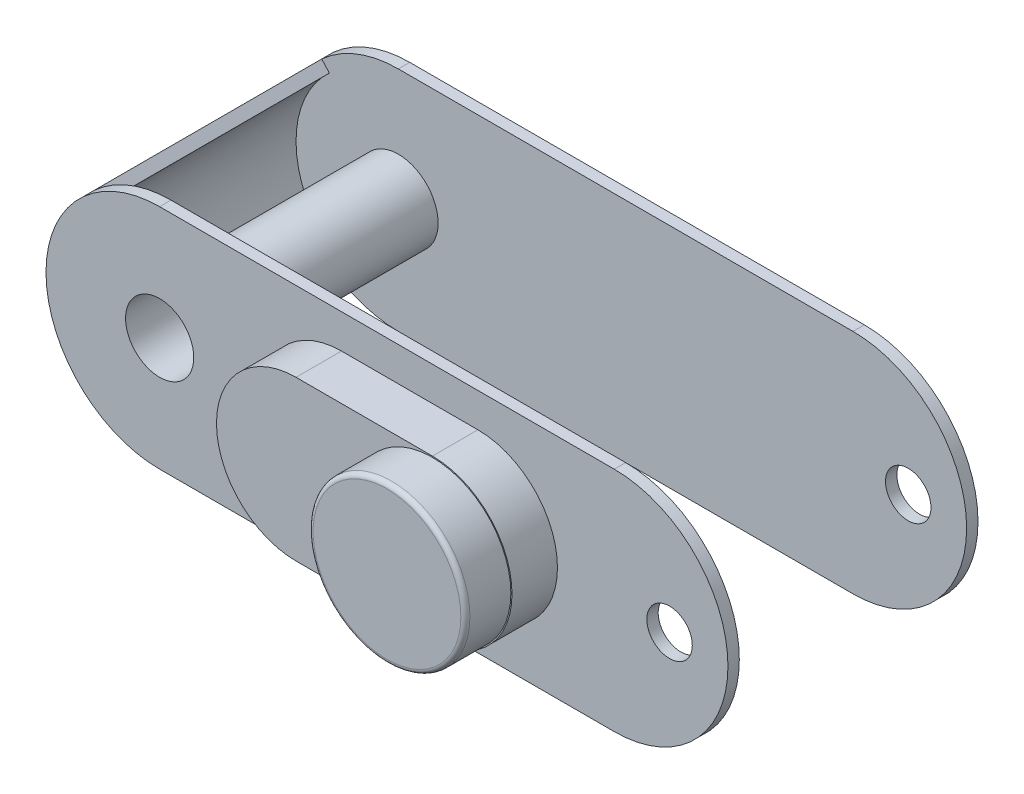
from build123d import *

# Parameters (mm, degrees)
SKETCH5_R           = 15
BOSS_EXTRUDE2_DEPTH = 5
BOSS_EXTRUDE3_START = 100
SKETCH6_R           = 15
BOSS_EXTRUDE3_DEPTH = 5
SKETCH7_R           = 17.5
SKETCH7_R_2         = 15
BOSS_EXTRUDE4_DEPTH = 100
SKETCH8_R           = 10
CUT_EXTRUDE1_DEPTH  = 46
BOSS_EXTRUDE5_DEPTH = 20
SKETCH10_R          = 34.5
BOSS_EXTRUDE6_DEPTH = 20
SKETCH11_R          = 10
CUT_EXTRUDE2_DEPTH  = 127
BOSS_EXTRUDE8_REACH = 295.3
FILLET1_R           = 2


with BuildPart() as part:
    # Sketch5 → Boss-Extrude2 (new body)
    with BuildSketch(Plane.XY):
        with BuildLine():
            Line((0, 50), (200, 50))
            ThreePointArc((200, 50), (250, 0), (200, -50))
            Line((200, -50), (0, -50))
            ThreePointArc((0, -50), (-50, 0), (0, 50))
        make_face()
        Circle(SKETCH5_R, mode=Mode.SUBTRACT)
    extrude(amount=BOSS_EXTRUDE2_DEPTH)



with BuildPart() as body_2:
    # Sketch6 → Boss-Extrude3 (new body)
    with BuildSketch(Plane.XY.offset(5).offset(BOSS_EXTRUDE3_START)):
        with BuildLine():
            Line((0, -50), (200, -50))
            ThreePointArc((200, -50), (250, 0), (200, 50))
            Line((200, 50), (0, 50))
            ThreePointArc((0, 50), (-50, 0), (0, -50))
        make_face()
        Circle(SKETCH6_R, mode=Mode.SUBTRACT)
    extrude(amount=BOSS_EXTRUDE3_DEPTH)


with BuildPart() as part_1:
    add(part.part)

    add(body_2.part)  # Boss-Extrude4 merges body 2
    # Sketch7 → Boss-Extrude4 (add)
    with BuildSketch(Plane.XY.offset(5)):
        Circle(SKETCH7_R)
        Circle(SKETCH7_R_2, mode=Mode.SUBTRACT)
    extrude(amount=BOSS_EXTRUDE4_DEPTH)

    # Sketch8 → Cut-Extrude1 (cut)
    with BuildSketch(Plane(origin=(0, 0, 105), x_dir=(-1, 0, 0), z_dir=(0, 0, -1))):
        with Locations((-80, 0)):
            Circle(SKETCH8_R)
        with Locations((-140, 0)):
            Circle(SKETCH8_R)
    extrude(amount=-CUT_EXTRUDE1_DEPTH, mode=Mode.SUBTRACT)

    # Sketch9 → Boss-Extrude5 (add)
    with BuildSketch(Plane.XY.offset(110)):
        with BuildLine():
            Line((80, 35), (140, 35))
            ThreePointArc((140, 35), (175, 0), (140, -35))
            Line((140, -35), (80, -35))
            ThreePointArc((80, -35), (45, 0), (80, 35))
        make_face()
    extrude(amount=BOSS_EXTRUDE5_DEPTH)

    # Sketch10 → Boss-Extrude6 (add)
    with BuildSketch(Plane.XY.offset(130)):
        with Locations((140, 0)):
            Circle(SKETCH10_R)
    extrude(amount=BOSS_EXTRUDE6_DEPTH)

    # Sketch11 → Cut-Extrude2 (cut)
    with BuildSketch(Plane(origin=(0, 0, 0), x_dir=(-1, 0, 0), z_dir=(0, 0, -1))):
        with Locations(Location((-224.307420274, 0, 0), (0, 0, 180))):
            Circle(SKETCH11_R)
    extrude(amount=-CUT_EXTRUDE2_DEPTH, mode=Mode.SUBTRACT)

    # Sketch13 → Boss-Extrude8 (add, up to next)
    with BuildSketch(Plane.XY.offset(5), mode=Mode.PRIVATE) as boss_extrude8_sk1:
        with BuildLine():
            Line((-33.713123493, 36.924589427), (-30.341811144, 33.232130484))
            ThreePointArc((-30.341811144, 33.232130484), (-44.79995187, 4.238432777), (-36.035736887, -26.952285005))
            Line((-36.035736887, -26.952285005), (-40.039707652, -29.946983339))
            ThreePointArc((-40.039707652, -29.946983339), (-49.777724301, 4.709369752), (-33.713123493, 36.924589427))
        make_face()
    boss_extrude8_tool1 = extrude(boss_extrude8_sk1.sketch, amount=BOSS_EXTRUDE8_REACH, mode=Mode.PRIVATE) - part_1.part
    add(boss_extrude8_tool1.solids().sort_by_distance((-32.542205, 34.608391, 5))[0])

    # Fillet1
    fillet1_edges = [part_1.edges().sort_by_distance(p)[0] for p in [
        (105.5, 0, 150),
    ]]
    fillet(fillet1_edges, radius=FILLET1_R)


solid = part_1.part
